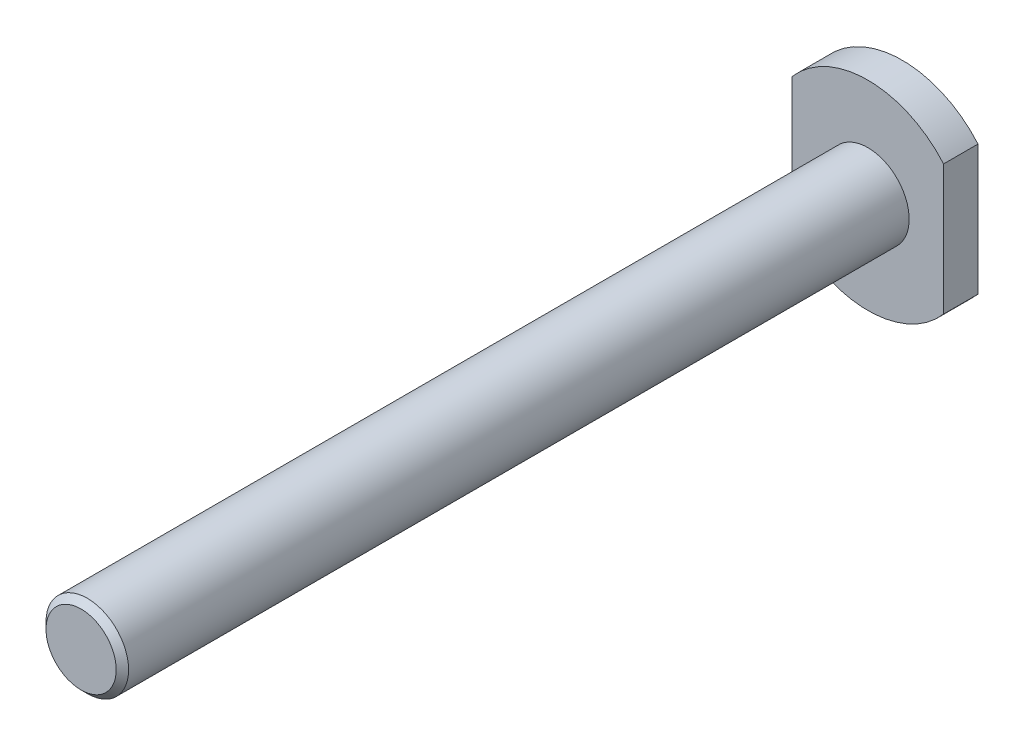
SolidWorks part; units mm, degrees
ref_plane "Front Plane" through (0, 0, 0) normal (0, 0, 1) x (1, 0, 0)
ref_plane "Top Plane" through (0, 0, 0) normal (0, 1, 0) x (1, 0, 0)
ref_plane "Right Plane" through (0, 0, 0) normal (1, 0, 0) x (0, 0, -1)
sketch "Sketch1" plane through (0, 0, 0) normal (0, 0, 1) x (1, 0, 0)
  circle A0 centre (0, 0) radius 6
extrude "Boss-Extrude1" add sketch "Sketch1" along normal blind 114.3
cosmetic thread "Cosmetic Thread2" parameters "D1"=80, "D2"=10.2
chamfer "Chamfer2" distance 0.9 angle 45 1 edges at (6, 0, 114.3)
sketch "Sketch2" plane through (0, 0, 0) normal (0, 0, -1) x (-1, 0, 0)
  line L1 (11, 9.4472) -> (11, -9.4472)
  line L2 (-11, 9.4472) -> (-11, -9.4472)
  arc A0 (-11, -9.4472) -> (11, -9.4472) centre (0, 0) ccw
  arc A1 (11, 9.4472) -> (-11, 9.4472) centre (0, 0) ccw
extrude "Boss-Extrude2" add sketch "Sketch2" along normal blind 5 contours A1 L2 A0 L1
sketch "Sketch4" plane through (0, 0, 0) normal (0, 1, 0) x (1, 0, 0)
  line L0 (0, -113.4) -> (0, 0) construction
  line L1 (0, -113.4) -> (0, -114.3) construction
  line L2 (-5.1, -114.3) -> (5.1, -114.3) construction
  point P0 (0, -69.5)
  dimension "D1" = 44.8
